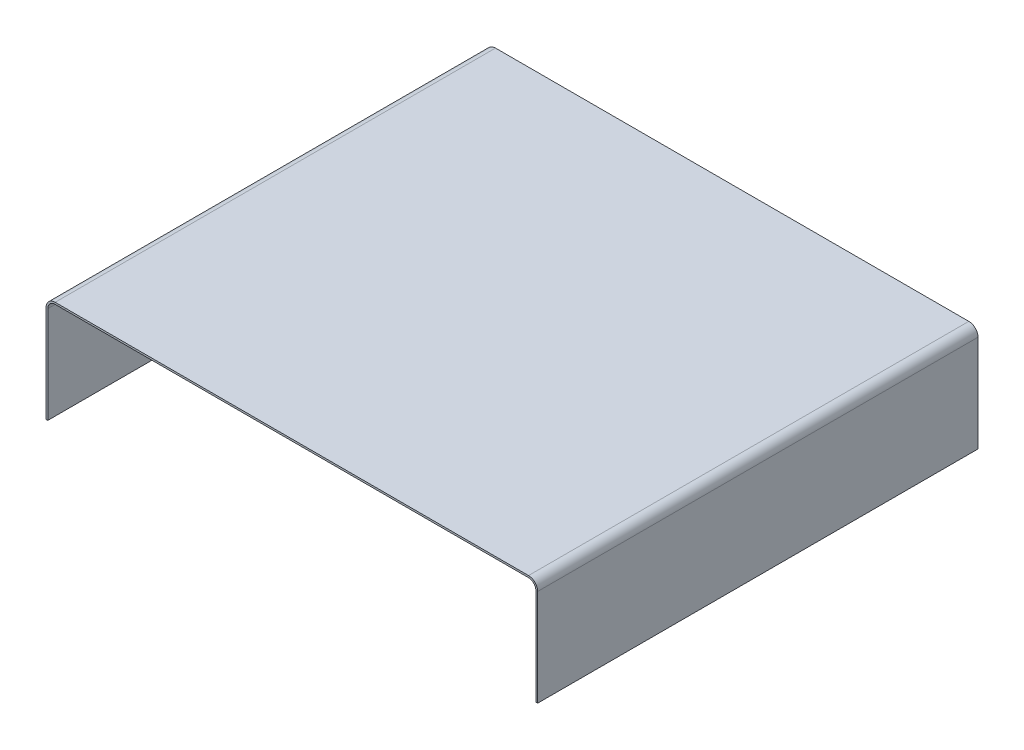
from build123d import *

# Parameters (mm, degrees)
EXTRUDE_THIN1_DEPTH = 480


with BuildPart() as part:
    # Sketch1 → Extrude-Thin1 (new body)
    with BuildSketch(Plane.XY):
        with BuildLine():
            Line((0, -115.5), (0, -10))
            ThreePointArc((0, -10), (2.928932188, -2.928932188), (10, 0))
            Line((10, 0), (526, 0))
            ThreePointArc((526, 0), (533.071067812, -2.928932188), (536, -10))
            Line((536, -10), (536, -115.5))
            Line((536, -115.5), (534, -115.5))
            Line((534, -115.5), (534, -10))
            ThreePointArc((534, -10), (531.656854249, -4.343145751), (526, -2))
            Line((526, -2), (10, -2))
            ThreePointArc((10, -2), (4.343145751, -4.343145751), (2, -10))
            Line((2, -10), (2, -115.5))
            Line((2, -115.5), (0, -115.5))
        make_face()
    extrude(amount=EXTRUDE_THIN1_DEPTH)


solid = part.part
